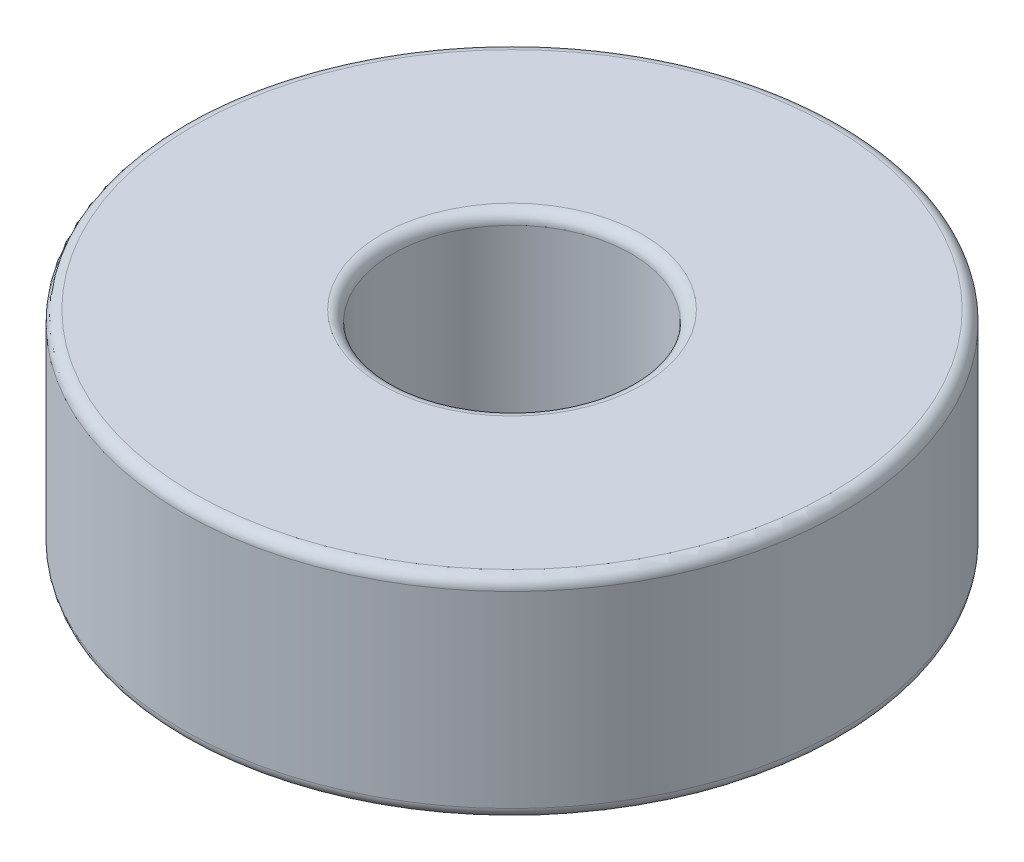
SolidWorks part; units mm, degrees
ref_plane "前视基准面" through (0, 0, 0) normal (0, 0, 1) x (1, 0, 0)
ref_plane "上视基准面" through (0, 0, 0) normal (0, 1, 0) x (1, 0, 0)
ref_plane "右视基准面" through (0, 0, 0) normal (1, 0, 0) x (0, 0, -1)
sketch "草图1" plane through (0, 0, 0) normal (0, 1, 0) x (1, 0, 0)
  circle A0 centre (0, 0) radius 23.5
  circle A1 centre (0, 0) radius 8.5
extrude "拉伸1" add sketch "草图1" along normal blind 15
fillet "圆角1" radius 0.8 4 edges at (0, 0, 8.5) (0, 0, 23.5) (0, 15, 8.5) (0, 15, 23.5)
